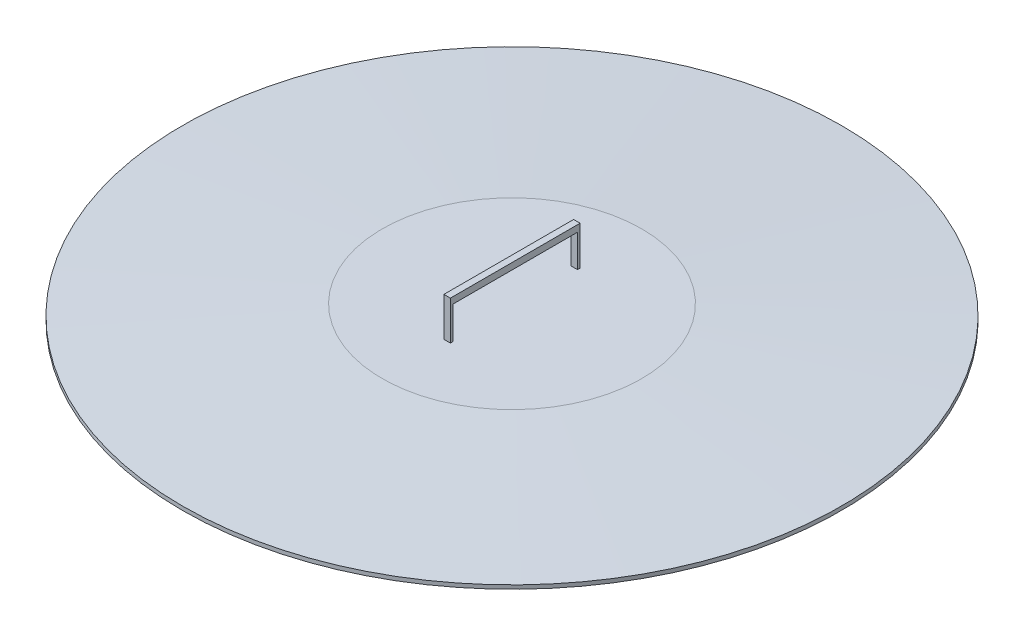
from build123d import *

# Parameters (mm, degrees)
BOSS_EXTRUDE2_DEPTH = 2.5


with BuildPart() as part:
    # Sketch1 → Revolve1 (revolve)
    with BuildSketch(Plane(origin=(0, 0, 0), x_dir=(0, 0, -1), z_dir=(1, 0, 0))):
        Polygon((253, -0.618600266), (253, 1.381399734), (99.973878508, 9.381399734), (0, 9.381399734), (0, 10.381399734), (100, 10.381399734), (254, 2.330486674), (254, 1.381399734), (254, -0.618600266), align=None)
    revolve(axis=Axis((0, 0, 0), (0, 1, 0)))

    # Sketch2 → Boss-Extrude2 (add, symmetric)
    with BuildSketch(Plane(origin=(0, 0, 0), x_dir=(0, 0, -1), z_dir=(1, 0, 0))):
        Polygon((-48, 10.381399734), (-48, 35.381399734), (48, 35.381399734), (48, 10.381399734), (50, 10.381399734), (50, 40.381399734), (-50, 40.381399734), (-50, 10.381399734), align=None)
    extrude(amount=BOSS_EXTRUDE2_DEPTH, both=True)


solid = part.part
